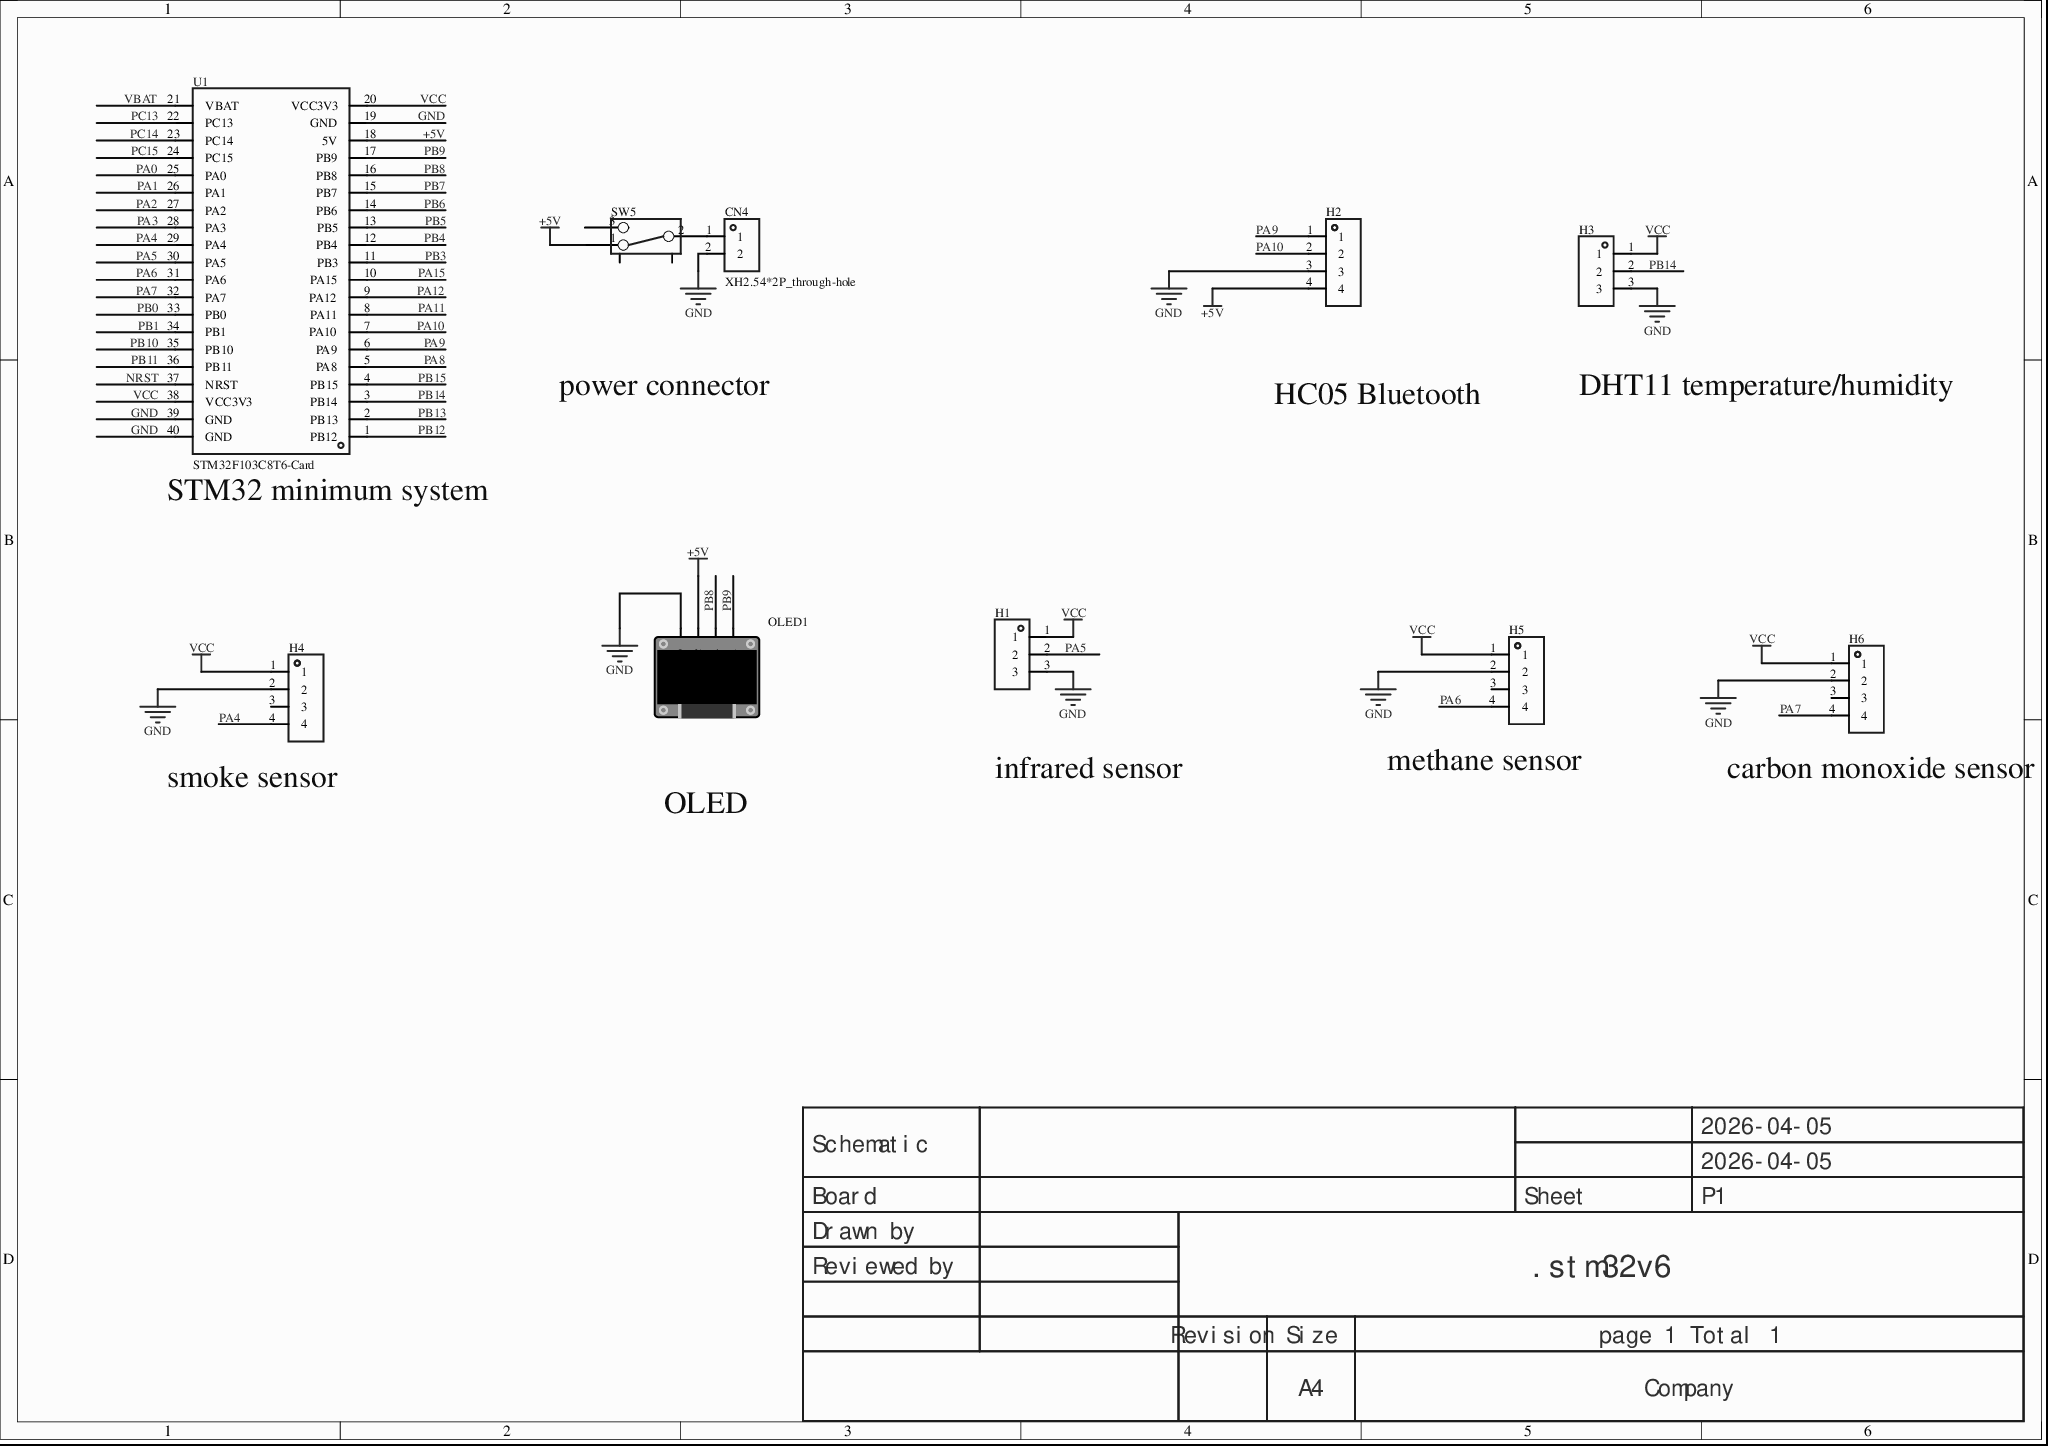
[diagram p0: MISC51056-3.schdoc]
# Altium project MISC51056-2.PrjPcb
1 sheet, 10 parts. Net scope: global (net labels, ports and power ports of the same name join across sheets).
Board file: MISC51056.pcbdoc

## Sheet MISC51056-3.schdoc
size 297 x 209 mm; Version: V1.0; @Project Name: MISC51056; @Page Count: 1; @Update Date: 2026-04-05; @Create Date: 2026-04-05; @Schematic Name: MISC51056; @Page No: 1; @Create Time: 23:22:16; @Update Time: 17:32:40; @Board Name: MISC51056

### Parts
CN4  XH2.54*2P_through-hole  [CONN-TH_2P-P2.50-XH2.54-2P]
H1  (no value)  [HDR-TH_3P-P2.54-V-F]
H2  (no value)  [HDR-TH_4P-P2.54-V-F]
H3  (no value)  [HDR-TH_3P-P2.54-V-F]
H4  (no value)  [HDR-TH_4P-P2.54-V-F]
H5  (no value)  [HDR-TH_4P-P2.54-V-F]
H6  (no value)  [HDR-TH_4P-P2.54-V-F]
OLED1  (no value)  [0.96OLED_4P]
SW5  (no value)  [拨动开关]
U1  STM32F103C8T6-Card  [CONN-TH_L53.3-W22.9_STM32F103C8T6-CARD]

### Nets
+5V: H2.4 OLED1.2(VCC) SW5.1 U1.18(5V)
GND: CN4.2 H1.3 H2.3 H3.3 H4.2 H5.2 H6.2 OLED1.1(GND) U1.19(GND) U1.39(GND) U1.40(GND)
VCC: H1.1 H3.1 H4.1 H5.1 H6.1 U1.20(VCC3V3) U1.38(VCC3V3)
NRST: U1.37(NRST)
PA0: U1.25(PA0)
PA1: U1.26(PA1)
PA2: U1.27(PA2)
PA3: U1.28(PA3)
PA4: H4.4 U1.29(PA4)
PA5: H1.2 U1.30(PA5)
PA6: H5.4 U1.31(PA6)
PA7: H6.4 U1.32(PA7)
PA8: U1.5(PA8)
PA9: H2.1 U1.6(PA9)
PA10: H2.2 U1.7(PA10)
PA11: U1.8(PA11)
PA12: U1.9(PA12)
PA15: U1.10(PA15)
PB0: U1.33(PB0)
PB1: U1.34(PB1)
PB3: U1.11(PB3)
PB4: U1.12(PB4)
PB5: U1.13(PB5)
PB6: U1.14(PB6)
PB7: U1.15(PB7)
PB8: OLED1.3(SCL) U1.16(PB8)
PB9: OLED1.4(SDA) U1.17(PB9)
PB10: U1.35(PB10)
PB11: U1.36(PB11)
PB12: U1.1(PB12)
PB13: U1.2(PB13)
PB14: H3.2 U1.3(PB14)
PB15: U1.4(PB15)
PC13: U1.22(PC13)
PC14: U1.23(PC14)
PC15: U1.24(PC15)
VBAT: U1.21(VBAT)
NetCN4_1: CN4.1 SW5.2

Not connected (* = marked no-connect by the designer): H4 3; H5 3; H6 3; SW5 3 4 5

### Notes on the sheet
- power connector
- HC05 Bluetooth
- DHT11 temperature/humidity
- (near U1) STM32 minimum system
- infrared sensor
- (near H5) methane sensor
- (near H6) carbon monoxide sensor
- (near H4) smoke sensor
- OLED
- Labels drawn without touching a wire or pin: VCC
- 2026-04-05
- Schematic
- Board
- Sheet
- P1
- Drawn by
- Reviewed by
- .stm32v6
- Revision
- Size
- A4
- page 1 Total 1
- Company

### Library data of the parts
CN4 = XH2.54*2P_直插: 3D Model: 325c595e30db4df8abe76612dd40b0fa0819f05c4eef4c71ace90d822a990e87; 3D Model Transform: 295.275,228.346,0,180,0,0,-0.002,-20.079,-137.795; AddInBom: yes; Symbol: XH2.54*2P_through-hole; Device: XH2.54*2P_through-hole; LCSC Part Name: XH2.54*2P_直插; Supplier Part: C9900008615; Manufacturer Part: XH2.54*2P_直插; Supplier Footprint: XH2.54_2P; JLCPCB Part Class: Extended Part; Supplier: LCSC; ConvertToPcb: yes; FootprintName: CONN-TH_2P-P2.50-XH2.54-2P; ModelName: CONN-TH_2P-P2.50-XH2.54-2P
H1 H3 = HDR-F_2.54_1x3P: Symbol: PM254V-11-03-H85; 3D Model: f3b3cc5aae9641bf9e56fc160cef875b; 3D Model Transform: 299.9994,100,0,0,0,0,0,0,-118.11; ConvertToPcb: yes; ModelName: HDR2.54-F-LI-1X3P; Device: HDR-F_2.54_1x3P; Supplier Part: C541850; Supplier Footprint: 插件; AddInBom: yes; FootprintName: HDR-TH_3P-P2.54-V-F
H2 H4 = HDR-F_2.54_1x4P: Symbol: 2.54-1*4P female; ConvertToPcb: yes; ModelId: d187812051054f85879fcaa51a310d8e0819f05c4eef4c71ace90d822a990e87; ModelTransform: 419.6842,98.464,0,0,0,0,0,0,-118.11; Device: HDR-F_2.54_1x4P; AddInBom: yes; SupplierPart: C2718488; Supplier Footprint: 插件; FootprintName: HDR-TH_4P-P2.54-V-F; ModelName: HDR-TH_4P-P2.54-V-F
H5 H6 = HDR-F_2.54_1x4P: Symbol: 2.54-1*4P female; 3D Model: d187812051054f85879fcaa51a310d8e0819f05c4eef4c71ace90d822a990e87; 3D Model Transform: 419.6842,98.464,0,0,0,0,0,0,-118.11; ConvertToPcb: yes; Device: HDR-F_2.54_1x4P; Supplier Part: C2718488; Supplier Footprint: 插件; AddInBom: yes; FootprintName: HDR-TH_4P-P2.54-V-F; ModelName: HDR-TH_4P-P2.54-V-F
OLED1 = 0.96OLED模块_4P: Symbol: 0.96OLED module_4P; ConvertToPcb: yes; ModelId: 79c000fdb68d45a296c2e9bedf4f9055; ModelTransform: 1393.69792,1318.895,0,0,0,0,0,-560.079,-137.795; Device: 0.96OLED module_4P; AddInBom: yes; FootprintName: 0.96OLED_4P; Supplier Footprint: 插件; ModelName: 0.96OLED_4P
SW5 = 拨动开关_正: Symbol: toggle switch; Device: toggle switch_upright; ConvertToPcb: yes; ModelId: 4321fe59a4074cbfb4989553f297c68f0819f05c4eef4c71ace90d822a990e87; ModelName: SW-TH_SS-12D02-VG4; ModelTransform: 370.09,208.7,472.35,0,0,0,0,0,-110; AddInBom: yes; Supplier Footprint: 插件; FootprintName: toggle switch
U1 = STM32F103C8T6-Card: AddInBom: yes; Symbol: STM32F103C8T6-CARD; Device: STM32F103C8T6-Card; LCSC Part Name: STM32F103C8T6-Card; SupplierPart: C9900077949; ManufacturerPart: STM32F103C8T6-Card; Supplier Footprint: 插件; Supplier: LCSC; ConvertToPcb: yes; FootprintName: CONN-TH_L53.3-W22.9_STM32F103C8T6-CARD